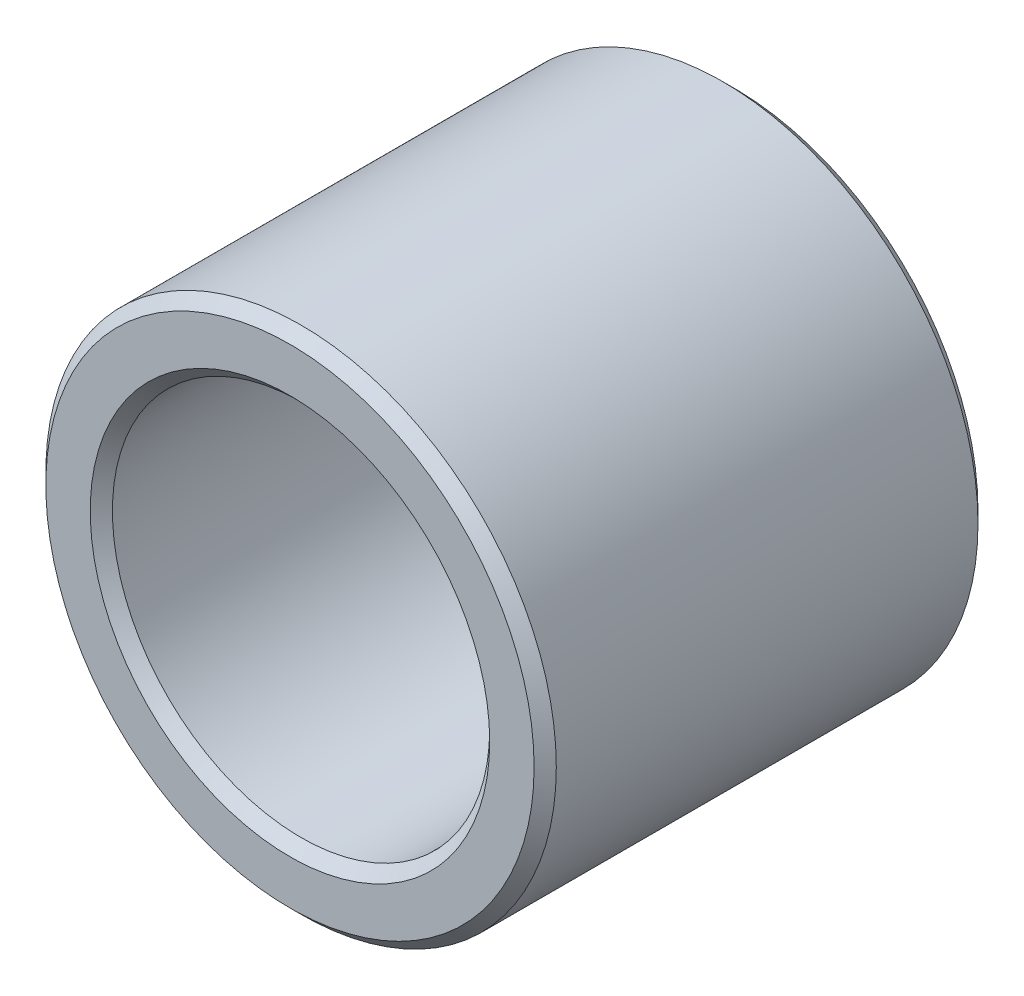
from build123d import *

# Parameters (mm, degrees)
SKETCH1_R           = 11.5
SKETCH1_R_2         = 8.5
BOSS_EXTRUDE1_DEPTH = 20
CHAMFER1_SIZE       = 0.5


with BuildPart() as part:
    # Sketch1 → Boss-Extrude1 (new body)
    with BuildSketch(Plane.XY):
        Circle(SKETCH1_R)
        Circle(SKETCH1_R_2, mode=Mode.SUBTRACT)
    extrude(amount=BOSS_EXTRUDE1_DEPTH)

    # Chamfer1
    chamfer1_edges = [part.edges().sort_by_distance(p)[0] for p in [
        (-11.5, 0, 0),
        (-11.5, 0, 20),
        (-8.5, 0, 0),
        (-8.5, 0, 20),
    ]]
    chamfer(chamfer1_edges, length=CHAMFER1_SIZE)


solid = part.part
